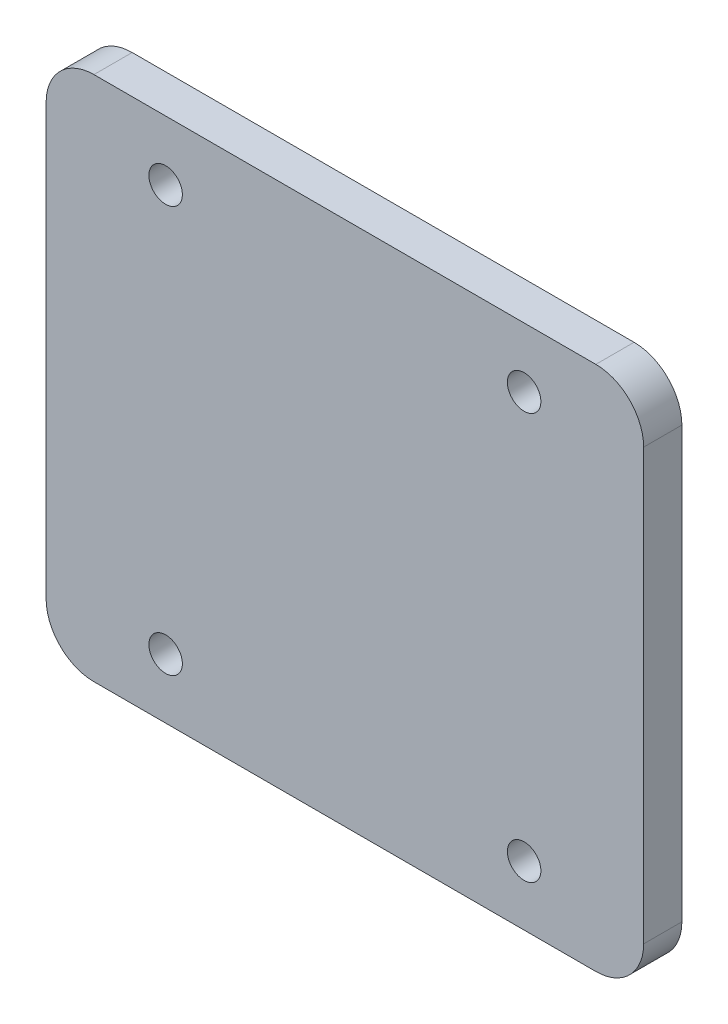
SolidWorks part; units mm, degrees
material "Q235B"
ref_plane "Front Plane" through (0, 0, 0) normal (0, 0, 1) x (1, 0, 0)
ref_plane "Top Plane" through (0, 0, 0) normal (0, 1, 0) x (1, 0, 0)
ref_plane "Right Plane" through (0, 0, 0) normal (1, 0, 0) x (0, 0, -1)
sketch "Sketch1" plane through (0, 0, 0) normal (0, 0, 1) x (1, 0, 0)
  line L1 (125, -110) -> (-125, -110)
  line L2 (125, -110) -> (125, 110)
  line L3 (125, 110) -> (-125, 110)
  line L4 (-125, -110) -> (-125, 110)
  line L5 (125, -110) -> (-125, 110) construction
  line L6 (125, 110) -> (-125, -110) construction
  point P0 (0, 0)
  dimension "D1" = 220
  dimension "D2" = 250
extrude "Boss-Extrude1" add sketch "Sketch1" along normal mid plane 16
hole_wizard "Ø14 Hole1" positions "Sketch2" profile "Sketch3" hole size "Ø18.0" standard "GB" end condition up to next
sketch "Sketch2" plane through (0, 0, 8) normal (0, 0, 1) x (1, 0, 0)
  line L0 (0, 110) -> (0, 0) construction
  line L1 (125, 110) -> (-125, 110) construction
  line L2 (0, 0) -> (-125, 0) construction
  line L3 (-125, 110) -> (-125, -110) construction
  point P0 (-75, 85)
  point P13 (75, 85)
  point P14 (75, -85)
  point P15 (-75, -85)
  dimension "D1" = 150
  dimension "D2" = 170
sketch "Sketch3" plane through (-75, 85, 8) normal (1, 0, 0) x (0, -1, 0)
  line L0 (0, 0) -> (0, 16)
  line L1 (0, 16) -> (7, 16)
  line L2 (7, 16) -> (7, 0)
  line L5 (7, 0) -> (0, 0)
  line L11 (0, -6.35) -> (0, 107.95) construction
  dimension "通孔孔直径" = 14
  dimension "通孔孔深度" = 16
chamfer "Chamfer1" [suppressed] distance 10 angle 45
fillet "Fillet2" radius 20 4 edges at (125, 110, 0) (125, -110, 0) (-125, -110, 0) (-125, 110, 0)
